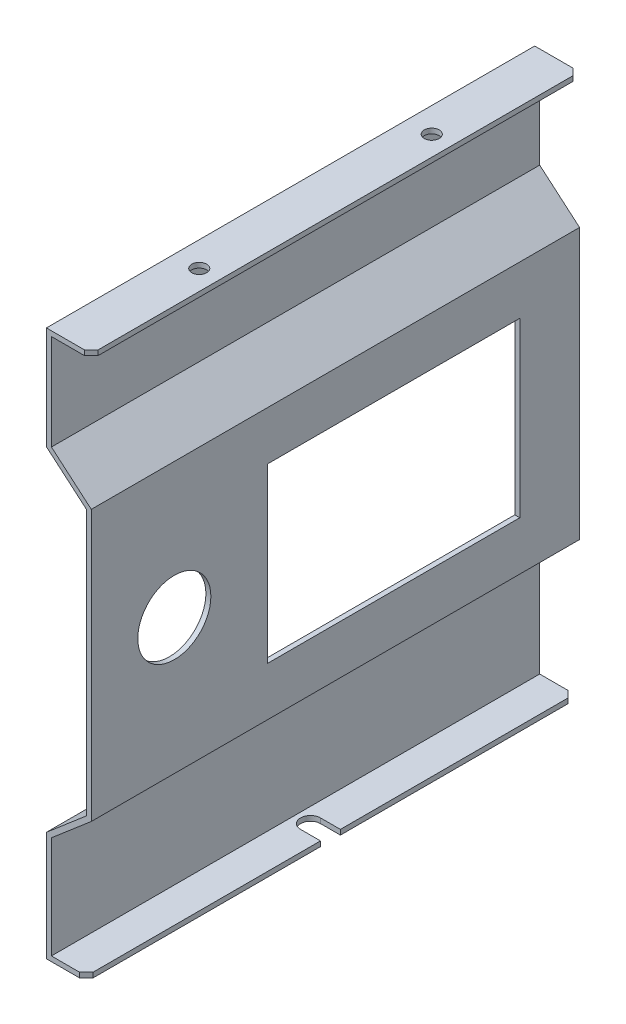
SolidWorks part; units mm, degrees
material "SPCC"
ref_plane "Front Plane" through (0, 0, 0) normal (0, 0, 1) x (1, 0, 0)
ref_plane "Top Plane" through (0, 0, 0) normal (0, 1, 0) x (1, 0, 0)
ref_plane "Right Plane" through (0, 0, 0) normal (1, 0, 0) x (0, 0, -1)
sketch "Sketch1" plane through (0, 0, 0) normal (0, 0, 1) x (1, 0, 0)
  line L0 (0, 0) -> (0, 33)
  line L1 (0, 33) -> (12, 43.249)
  line L2 (12, 43.249) -> (12, 123.249)
  line L3 (12, 123.249) -> (0, 133.4979)
  line L4 (0, 133.4979) -> (0, 164.4979)
  line L5 (0, 164.4979) -> (13.5, 164.4979)
  line L6 (0, 0) -> (12, 0)
  dimension "D1" = 33
  dimension "D2" = 130.5
  dimension "D3" = 80
  dimension "D4" = 12
  dimension "D5" = 130.5
  dimension "D6" = 31
  dimension "D7" = 12
  dimension "D8" = 12
  dimension "D9" = 13.5
extrude "Extrude-Thin1" add sketch "Sketch1" along normal mid plane 147 thin
sketch "Sketch2" plane through (12, 0, 0) normal (-1, 0, 0) x (0, 0, 1)
  line L0 (0, 0) -> (0, 162.0492) construction
  line L1 (-55.5, 109.249) -> (20.5, 109.249)
  line L2 (-55.5, 109.249) -> (-55.5, 57.249)
  line L3 (-55.5, 57.249) -> (20.5, 57.249)
  line L4 (20.5, 109.249) -> (20.5, 57.249)
  line L5 (73.5, 43.249) -> (-73.5, 43.249) construction
  line L6 (-73.5, 123.249) -> (-73.5, 43.249) construction
  dimension "D1" = 76
  dimension "D2" = 52
  dimension "D3" = 18
  dimension "D4" = 14
extrude "Cut-Extrude1" cut sketch "Sketch2" against normal blind 10
chamfer "Chamfer1" distance 2 angle 45 4 edges at (13.5, 163.7479, -73.5) (13.5, 163.7479, 73.5) (12, 0.75, -73.5) (12, 0.75, 73.5)
sketch "Sketch6" plane through (0, 0, 0) normal (0, -1, 0) x (1, 0, 0)
  line L0 (6, 0) -> (12, 0) construction
  line L1 (12, 71.5) -> (12, -71.5) construction
  line L2 (6, 3) -> (12, 3)
  line L3 (6, -3) -> (12, -3)
  arc A0 (6, 3) -> (6, -3) centre (6, 0) ccw
  arc A1 (12, -3) -> (12, 3) centre (12, 0) ccw
  point P4 (9, 0)
  dimension "D1" = 6
  dimension "D2" = 6
extrude "Cut-Extrude3" cut sketch "Sketch6" against normal blind 5
sketch "Sketch7" plane through (12, 0, 0) normal (-1, 0, 0) x (0, 0, 1)
  line L0 (73.5, 123.249) -> (73.5, 43.249) construction
  line L1 (20.5, 83.249) -> (88.4738, 83.249) construction
  line L2 (20.5, 57.249) -> (20.5, 109.249) construction
  circle A0 centre (48.5, 83.249) radius 11
  dimension "D1" = 22
  dimension "D2" = 25
extrude "Cut-Extrude4" cut sketch "Sketch7" against normal blind 10
sketch "Sketch8" plane through (0, 164.4979, 0) normal (0, 1, 0) x (1, 0, 0)
  line L0 (0, 0) -> (21.0538, 0) construction
  line L1 (8.5, 40) -> (6.5, 40) construction
  line L2 (8.5, 40) -> (8.5, 30) construction
  line L3 (8.5, 30) -> (6.5, 30) construction
  line L4 (6.5, 40) -> (6.5, 30) construction
  line L5 (8.5, 40) -> (6.5, 30) construction
  line L6 (8.5, 30) -> (6.5, 40) construction
  line L7 (13.5, -71.5) -> (13.5, 71.5) construction
  circle A0 centre (7.5, 35) radius 2.25
  point P0 (7.5, 35)
  dimension "D5" = 4.5
  dimension "D1" = 10
  dimension "D2" = 2
  dimension "D3" = 6
  dimension "D4" = 35
extrude "Cut-Extrude5" cut sketch "Sketch8" against normal blind 10
mirror "Mirror1" about plane through (0, 0, 0) normal (0, 0, 1) of "Cut-Extrude5"
